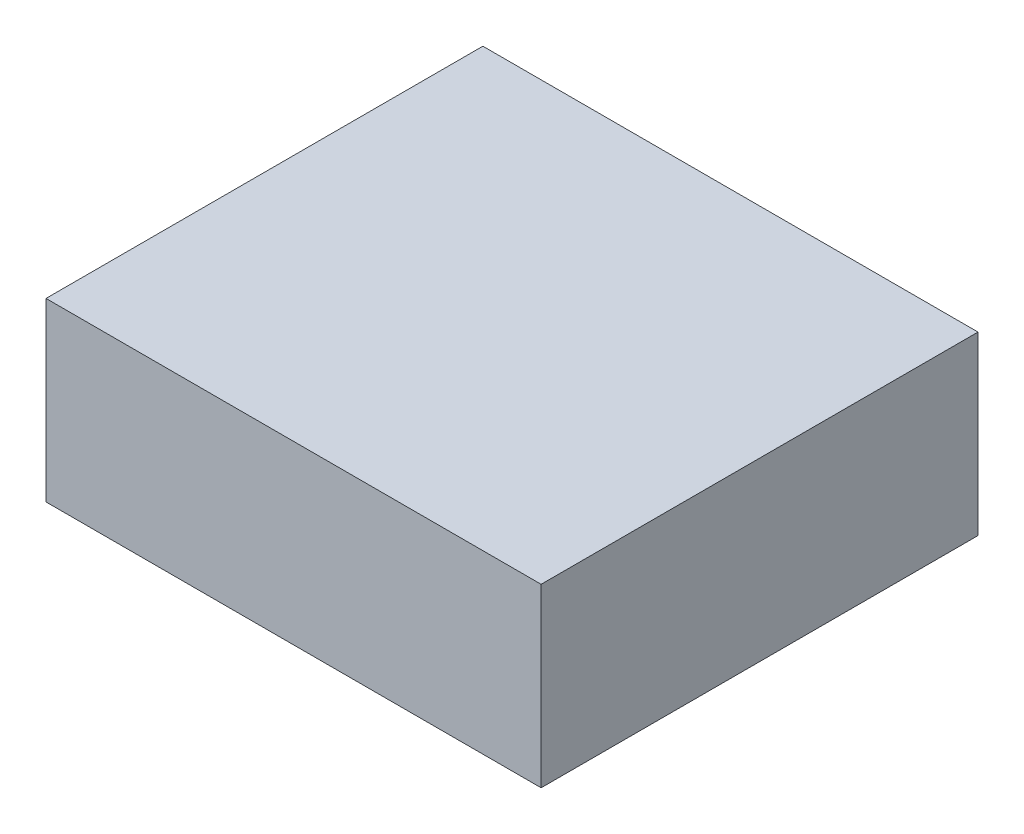
from build123d import *

# Parameters (mm, degrees)
SKETCH_1_W          = 170
SKETCH_1_H          = 60.52
EXTRUDE_1_DEPTH     = 150
SKETCH_2_W          = 150
SKETCH_2_H          = 130
CUT_EXTRUDE_1_DEPTH = 50.52


with BuildPart() as part:
    # 草图1 → 凸台-拉伸1 (new body)
    with BuildSketch(Plane.XY):
        with Locations((-32.516262295, 4.960655738)):
            Rectangle(SKETCH_1_W, SKETCH_1_H)
    extrude(amount=EXTRUDE_1_DEPTH)

    # 草图2 → 切除-拉伸1 (cut)
    with BuildSketch(Plane.XZ.offset(25.299344262)):
        with Locations((-32.516262295, 75)):
            Rectangle(SKETCH_2_W, SKETCH_2_H)
    extrude(amount=-CUT_EXTRUDE_1_DEPTH, mode=Mode.SUBTRACT)


solid = part.part
